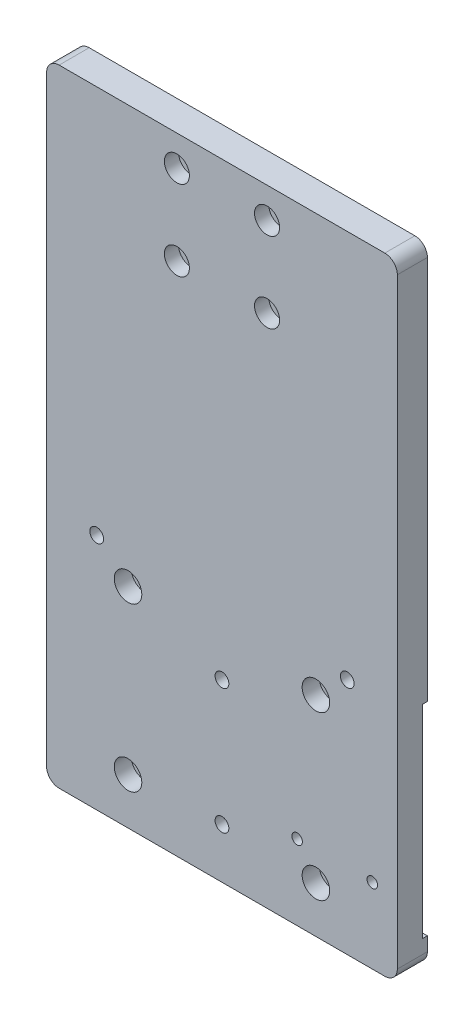
SolidWorks part; units mm, degrees
ref_plane "前视基准面" through (0, 0, 0) normal (0, 0, 1) x (1, 0, 0)
ref_plane "上视基准面" through (0, 0, 0) normal (0, 1, 0) x (1, 0, 0)
ref_plane "右视基准面" through (0, 0, 0) normal (1, 0, 0) x (0, 0, -1)
sketch "草图1" plane through (0, 0, 0) normal (0, 0, 1) x (1, 0, 0)
  line L1 (70, -125) -> (-70, -125)
  line L2 (70, -125) -> (70, 125)
  line L3 (70, 125) -> (-70, 125)
  line L4 (-70, -125) -> (-70, 125)
  line L5 (70, -125) -> (-70, 125) construction
  line L6 (70, 125) -> (-70, -125) construction
  point P0 (0, 0)
  dimension "D1" = 140
  dimension "D2" = 250
extrude "凸台-拉伸1" add sketch "草图1" along normal blind 12
hole_wizard "打孔尺寸(%根据)内六角圆柱头螺钉的类型1" positions "草图2" profile "草图3" counterbore size "M5" standard "GB"
sketch "草图2" plane through (0, 0, 12) normal (0, 0, 1) x (1, 0, 0)
  point P0 (-18, 112.8)
  point P3 (-18, 80.8)
  point P6 (18, 80.8)
  point P9 (18, 112.8)
sketch "草图3" plane through (-18, 112.8, 12) normal (1, 0, 0) x (0, -1, 0)
  line L0 (0, 0) -> (0, 16.6524)
  line L1 (0, 16.6524) -> (2.75, 15)
  line L2 (2.75, 15) -> (2.75, 5.7)
  line L3 (2.75, 5.7) -> (5, 5.7)
  line L4 (5, 5.7) -> (5, 0)
  line L5 (5, 0) -> (0, 0)
  line L10 (0, 16.6524) -> (-2.75, 15) construction
  line L11 (0, -6.35) -> (0, 107.95) construction
  dimension "孔直径" = 5.5
  dimension "孔深度" = 15
  dimension "柱形沉头孔直径" = 10
  dimension "柱形沉头孔深度" = 5.7
  dimension "导头角度" = 118
hole_wizard "打孔尺寸(%根据)内六角圆柱头螺钉的类型2" positions "草图4" profile "草图5" counterbore size "M6" standard "GB"
sketch "草图4" plane through (0, 0, 12) normal (0, 0, 1) x (1, 0, 0)
  point P0 (37.5, -106.5)
  point P3 (-37.5, -106.5)
  point P6 (-37.5, -41.5)
  point P9 (37.5, -41.5)
sketch "草图5" plane through (37.5, -106.5, 12) normal (1, 0, 0) x (0, -1, 0)
  line L0 (0, 0) -> (0, 16.9828)
  line L1 (0, 16.9828) -> (3.3, 15)
  line L2 (3.3, 15) -> (3.3, 6.8)
  line L3 (3.3, 6.8) -> (5.5, 6.8)
  line L4 (5.5, 6.8) -> (5.5, 0)
  line L5 (5.5, 0) -> (0, 0)
  line L10 (0, 16.9828) -> (-3.3, 15) construction
  line L11 (0, -6.35) -> (0, 107.95) construction
  dimension "孔直径" = 6.6
  dimension "孔深度" = 15
  dimension "柱形沉头孔直径" = 11
  dimension "柱形沉头孔深度" = 6.8
  dimension "导头角度" = 118
hole_wizard "打孔尺寸(%根据)内六角圆柱头螺钉的类型3" positions "草图6" profile "草图7" counterbore size "M5" standard "GB"
sketch "草图6" plane through (0, 0, 0) normal (0, 0, -1) x (-1, 0, 0)
  point P0 (0, -105)
  point P3 (0, -55)
sketch "草图7" plane through (0, -105, 0) normal (1, 0, 0) x (0, 1, 0)
  line L0 (0, 0) -> (0, 16.0524)
  line L1 (0, 16.0524) -> (2.75, 14.4)
  line L2 (2.75, 14.4) -> (2.75, 5.7)
  line L3 (2.75, 5.7) -> (5, 5.7)
  line L4 (5, 5.7) -> (5, 0)
  line L5 (5, 0) -> (0, 0)
  line L10 (0, 16.0524) -> (-2.75, 14.4) construction
  line L11 (0, -6.35) -> (0, 107.95) construction
  dimension "孔直径" = 5.5
  dimension "孔深度" = 14.4
  dimension "柱形沉头孔直径" = 10
  dimension "柱形沉头孔深度" = 5.7
  dimension "导头角度" = 118
sketch "草图8" plane through (0, 0, 0) normal (0, 0, -1) x (-1, 0, 0)
  line L0 (37.5, -106.5) -> (-37.5, -106.5) construction
  line L1 (-37.5, -41.5) -> (37.5, -41.5) construction
  line L2 (0, -41.5) -> (0, -106.5) construction
  line L3 (-70, -125) -> (-70, 125) construction
  line L4 (70, -114.5) -> (-70, -114.5)
  line L5 (70, -114.5) -> (70, -33.5)
  line L6 (70, -33.5) -> (-70, -33.5)
  line L7 (-70, -114.5) -> (-70, -33.5)
  line L8 (70, -114.5) -> (-70, -33.5) construction
  line L9 (70, -33.5) -> (-70, -114.5) construction
  point P10 (0, -74)
  dimension "D1" = 81
extrude "切除-拉伸1" cut sketch "草图8" against normal blind 2
hole_wizard "打孔尺寸(%根据)内六角圆柱头螺钉的类型0" positions "草图9" profile "草图10" counterbore size "M5" standard "GB" end condition up to next
sketch "草图9" plane through (0, 0, 0) normal (0, 0, -1) x (-1, 0, 0)
  point P0 (-50, -30)
  point P3 (50, -30)
sketch "草图10" plane through (50, -30, 0) normal (1, 0, 0) x (0, 1, 0)
  line L0 (0, 0) -> (0, 12)
  line L1 (0, 12) -> (2.75, 12)
  line L3 (2.75, 12) -> (2.75, 7)
  line L4 (2.75, 7) -> (5, 7)
  line L5 (5, 7) -> (5, 0)
  line L7 (5, 0) -> (0, 0)
  line L11 (0, -6.35) -> (0, 107.95) construction
  dimension "通孔孔直径" = 5.5
  dimension "通孔孔深度" = 12
  dimension "柱形沉头孔直径" = 10
  dimension "柱形沉头孔深度" = 7
hole_wizard "M5 螺纹孔1" positions "草图11" profile "草图12" tap size "M5" standard "GB" end condition up to next
sketch "草图11" plane through (0, 0, 12) normal (0, 0, 1) x (1, 0, 0)
  line L0 (27, -95) -> (33, -95) construction
  line L1 (27, -90) -> (27, -100) construction
  line L2 (33, -100) -> (33, -90) construction
  line L5 (57, -95) -> (63, -95) construction
  line L6 (57, -90) -> (57, -100) construction
  line L7 (63, -100) -> (63, -90) construction
  point P0 (30, -95)
  point P2 (60, -95)
sketch "草图12" plane through (30, -95, 12) normal (1, 0, 0) x (0, -1, 0)
  line L0 (0, 0) -> (0, 10)
  line L1 (0, 10) -> (2.1, 10)
  line L2 (2.1, 10) -> (2.1, 0)
  line L5 (2.1, 0) -> (0, 0)
  line L11 (0, -6.35) -> (0, 107.95) construction
  dimension "通孔螺纹孔钻头直径" = 4.2
  dimension "通孔螺纹孔钻头深度" = 10
cosmetic thread "孔螺蚊线2" parameters "D2"=5
cosmetic thread "孔螺蚊线3" parameters "D2"=5
fillet "圆角1" radius 5 4 edges at (-70, 125, 6) (70, 125, 6) (-70, -125, 6) (70, -125, 6)
